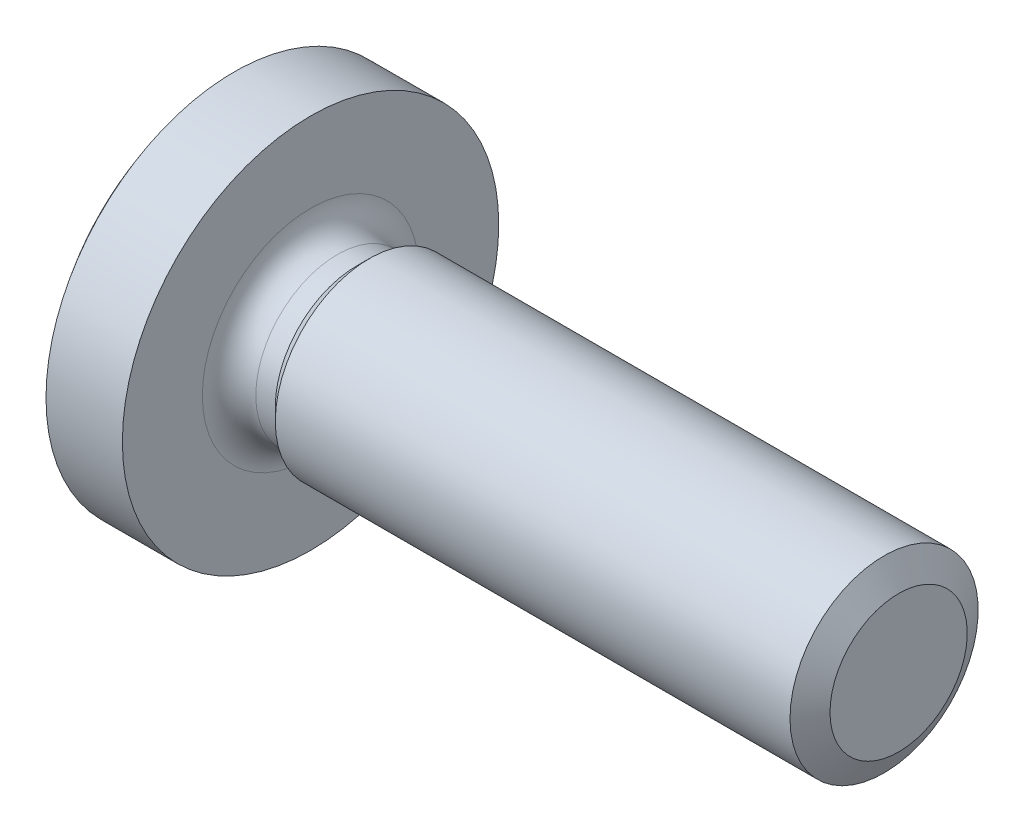
SolidWorks part; units mm, degrees
revolve "基体-旋转" add sketch "草图2" angle 360 about L0
sketch "草图2" plane through (0, 0, 0) normal (0, 0, 1) x (1, 0, 0)
  line L0 (-1.3318, 0) -> (6.5885, 0) construction
  line L1 (0, 0) -> (31, 0)
  line L2 (31, 0) -> (31, 4)
  line L3 (31, 4) -> (8.5, 4)
  line L4 (8.5, 4) -> (7.964, 3.464)
  line L5 (7.964, 3.464) -> (7.136, 3.464)
  line L6 (6, 4.6) -> (6, 8)
  line L7 (6, 8) -> (2.753, 8)
  arc A0 (6, 4.6) -> (7.136, 3.464) centre (7.136, 4.6) ccw
  arc A1 (0, 0) -> (2.753, 8) centre (13, 0) cw
cosmetic thread "装饰螺纹线1" parameters "D1"=22.5, "D2"=6.928
material "钢"
ref_plane "前视" through (0, 0, 0) normal (0, 0, 1) x (1, 0, 0)
ref_plane "上视" through (0, 0, 0) normal (0, 1, 0) x (1, 0, 0)
ref_plane "右视" through (0, 0, 0) normal (1, 0, 0) x (0, 0, -1)
sketch "尺寸草图" plane through (0, 0, 0) normal (0, 0, 1) x (1, 0, 0)
  line L0 (0, 0) -> (25, 0)
  line L1 (0, 0) -> (0, 16)
  line L2 (25, 0) -> (25, 9.2)
  point P5 (0, 8)
  point P6 (23.75, 0)
  point P7 (2.5, 0)
  point P8 (6, 0)
  point P9 (12, 0)
  point P10 (9, 0)
  point P11 (20.4, 0)
sketch "草图3" plane through (0, 0, 0) normal (0, 0, 1) x (1, 0, 0)
  line L0 (30.3818, 4) -> (31.6318, 4)
  line L1 (31.6318, 4) -> (31, 2.9175)
  line L2 (31, 2.9175) -> (30.3818, 4)
  line L3 (31, 4) -> (8.5, 4) construction
  line L4 (31, -4) -> (31, 4) construction
  line L5 (-0.2428, 0) -> (7.1644, 0) construction
  line L6 (-1.3318, 0) -> (6.5885, 0) construction
revolve "切除-旋转1" cut sketch "草图3" angle 360 about L5
sketch "草图5" plane through (0, 0, 0) normal (1, 0, 0) x (0, 0, -1)
  line L1 (0.625, 4.5) -> (-0.625, 4.5)
  line L2 (0.625, 4.5) -> (0.625, -4.5)
  line L3 (0.625, -4.5) -> (-0.625, -4.5)
  line L4 (-0.625, 4.5) -> (-0.625, -4.5)
  point P4 (0.625, 0)
  point P5 (0, 4.5)
ref_plane "基准面1" through (4.6, 0, 0) normal (1, 0, 0) x (0, 0, -1)
pattern_linear "阵列(线性)1" [suppressed] count 19 spacing 1.25 along (1, 0, 0)
sketch "草图6" plane through (4.6, 0, 0) normal (1, 0, 0) x (0, 0, -1)
  point P0 (0, 0)
loft "切除-放样1" cut profiles "草图6", "草图5"
ref_plane "基准面2" through (0, 0, 0) normal (0, -0.7071, 0.7071) x (1, 0, 0)
mirror "镜向1" about plane through (0, 0, 0) normal (0, -0.7071, 0.7071) of "切除-放样1"
equation "\"l@草图2\" = \"l@尺寸草图\""
equation "\"dk@草图2\" = \"dk@尺寸草图\""
equation "\"k@草图2\" = \"k@尺寸草图\""
equation "\"D2@草图2\" = \"d@尺寸草图\"*0.866"
equation "\"a@草图2\" = \"a@尺寸草图\""
equation "\"D3@草图2\" = \"rf@尺寸草图\""
equation "\"d@草图2\" = \"d@尺寸草图\""
equation "\"da@草图2\" = \"da@尺寸草图\""
equation "\"D2@装饰螺纹线1\" = \"d@尺寸草图\"*0.866"
equation "\"D1@装饰螺纹线1\" = \"l@尺寸草图\"-\"a@尺寸草图\""
equation "\"P@草图3\" = \"P@尺寸草图\""
equation "\"D1@草图3\" = \"P@尺寸草图\"*0.866"
equation "\"h@基准面1\" = \"h@尺寸草图\""
equation "\"D1@草图5\" = \"P@尺寸草图\""
equation "\"m@草图5\" = \"m@尺寸草图\""
equation "\"D3@阵列(线性)1\" = \"P@尺寸草图\""
equation "\"D1@阵列(线性)1\" = (\"l@尺寸草图\"-\"a@尺寸草图\")/\"P@尺寸草图\"+1"
